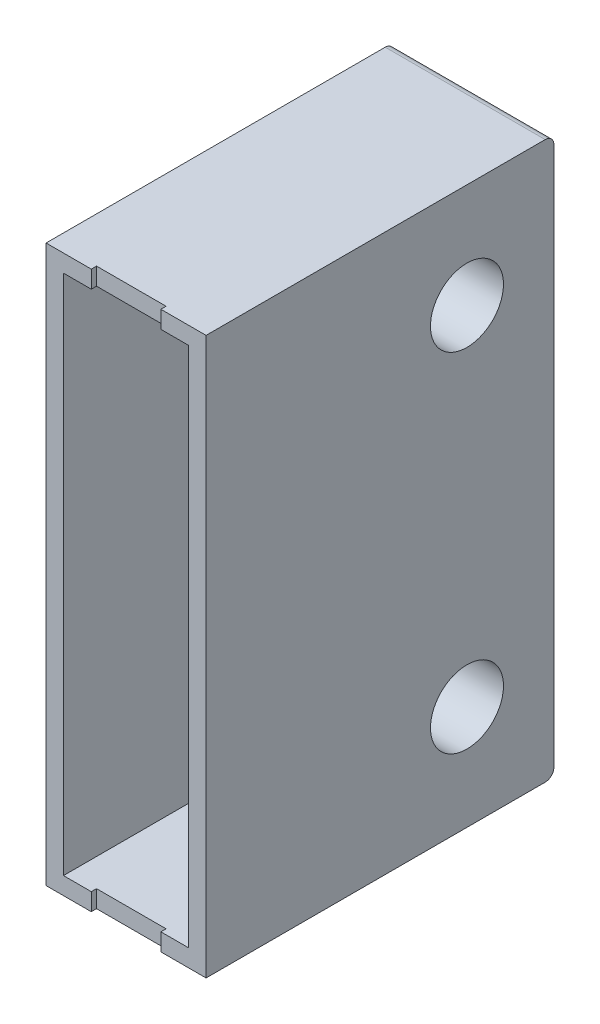
SolidWorks part; units mm, degrees
ref_plane "Front Plane" through (0, 0, 0) normal (0, 0, 1) x (1, 0, 0)
ref_plane "Top Plane" through (0, 0, 0) normal (0, 1, 0) x (1, 0, 0)
ref_plane "Right Plane" through (0, 0, 0) normal (1, 0, 0) x (0, 0, -1)
sketch "Sketch1" plane through (0, 0, 0) normal (0, 1, 0) x (1, 0, 0)
  line L0 (2, -10) -> (4.6, -10)
  line L1 (-4.6, -10) -> (-2, -10)
  line L2 (-4.6, -10) -> (-4.6, 10)
  line L3 (-4.6, 10) -> (4.6, 10)
  line L4 (4.6, -10) -> (4.6, 10)
  line L5 (-4.6, -10) -> (4.6, 10) construction
  line L6 (-4.6, 10) -> (4.6, -10) construction
  line L8 (-2, -10) -> (-2, -9.7)
  line L9 (-2, -9.7) -> (2, -9.7)
  line L10 (2, -10) -> (2, -9.7)
  point P0 (0, 0)
  dimension "D1" = 9.2
  dimension "D2" = 20
  dimension "D3" = 4
  dimension "D4" = 2
  dimension "D5" = 0.3
extrude "Boss-Extrude1" add sketch "Sketch1" along normal blind 32
sketch "Sketch2" plane through (4.6, 0, 0) normal (1, 0, 0) x (0, 0, -1)
  line L1 (-10, 0) -> (10, 0) construction
  line L2 (10, 32) -> (10, 0) construction
  circle A0 centre (5, 26) radius 2.1
  circle A1 centre (5, 6) radius 2.1
  dimension "D1" = 4.2
  dimension "D2" = 4.2
  dimension "D3" = 20
  dimension "D6" = 5
  dimension "D4" = 6
  dimension "D5" = 5
extrude "Cut-Extrude1" cut sketch "Sketch2" against normal through all
sketch "Sketch3" plane through (0, 0, -10) normal (0, 0, -1) x (-1, 0, 0)
  circle A0 centre (0, 18.9619) radius 1.7409
extrude "Boss-Extrude2" add sketch "Sketch3" along normal blind 0.1
sketch "Sketch4" plane through (0, 0, 0) normal (0, -1, 0) x (1, 0, 0)
  circle A0 centre (0, 0) radius 3.5
  dimension "D1" = 7
extrude "Boss-Extrude3" add sketch "Sketch4" along normal blind 4
sketch "Sketch5" plane through (0, -4, 0) normal (0, -1, 0) x (1, 0, 0)
  circle A0 centre (0, 0) radius 2.5
  dimension "D1" = 5
extrude "Boss-Extrude4" add sketch "Sketch5" along normal blind 62
fillet "Fillet1" radius 0.2 1 edges at (0, -4, -3.5)
fillet "Fillet2" radius 0.5 2 edges at (0, 0, -10) (0, 32, -10)
sketch "Sketch6" plane through (0, 0, 10) normal (0, 0, 1) x (1, 0, 0)
  line L0 (2, 32) -> (4.6, 32) construction
  line L1 (-3.6, 31) -> (3.6, 31)
  line L2 (-3.6, 31) -> (-3.6, 1)
  line L3 (-3.6, 1) -> (3.6, 1)
  line L4 (3.6, 31) -> (3.6, 1)
  line L5 (4.6, 32) -> (4.6, 0) construction
  line L6 (2, 0) -> (4.6, 0) construction
  line L7 (-4.6, 32) -> (-4.6, 0) construction
  dimension "D1" = 1
  dimension "D2" = 1
  dimension "D3" = 1
  dimension "D4" = 1
extrude "Cut-Extrude2" cut sketch "Sketch6" against normal blind 19
sketch "Sketch7" plane through (0, 0, 0) normal (0, -1, 0) x (1, 0, 0)
  line L1 (4.0388, 6.0151) -> (-12.2329, 6.0151)
  line L2 (4.0388, 6.0151) -> (4.0388, -17.6148)
  line L3 (4.0388, -17.6148) -> (-12.2329, -17.6148)
  line L4 (-12.2329, 6.0151) -> (-12.2329, -17.6148)
extrude "Cut-Extrude3" cut sketch "Sketch7" along normal blind 74.5
sketch "Sketch8" plane through (0, 0, 0) normal (0, -1, 0) x (1, 0, 0)
  line L0 (2, 10) -> (4.6, 10) construction
  circle A0 centre (0, 0) radius 1.9
  dimension "D1" = 3.8
  dimension "D2" = 10
extrude "Cut-Extrude4" cut sketch "Sketch8" against normal blind 17.5
sketch "Sketch9" plane through (3.6, 0, 0) normal (-1, 0, 0) x (0, 0, 1)
  circle A0 centre (-5, 26) radius 2.1
  circle A1 centre (-5, 26) radius 3.1
  circle A3 centre (-5, 6) radius 2.1
  circle A4 centre (-5, 6) radius 3.1
  dimension "D1" = 6.2
  dimension "D2" = 6.2
extrude "Boss-Extrude5" add sketch "Sketch9" along normal up to surface (7.2 mm away) up to face at (-3.6, 23.9, -5)
